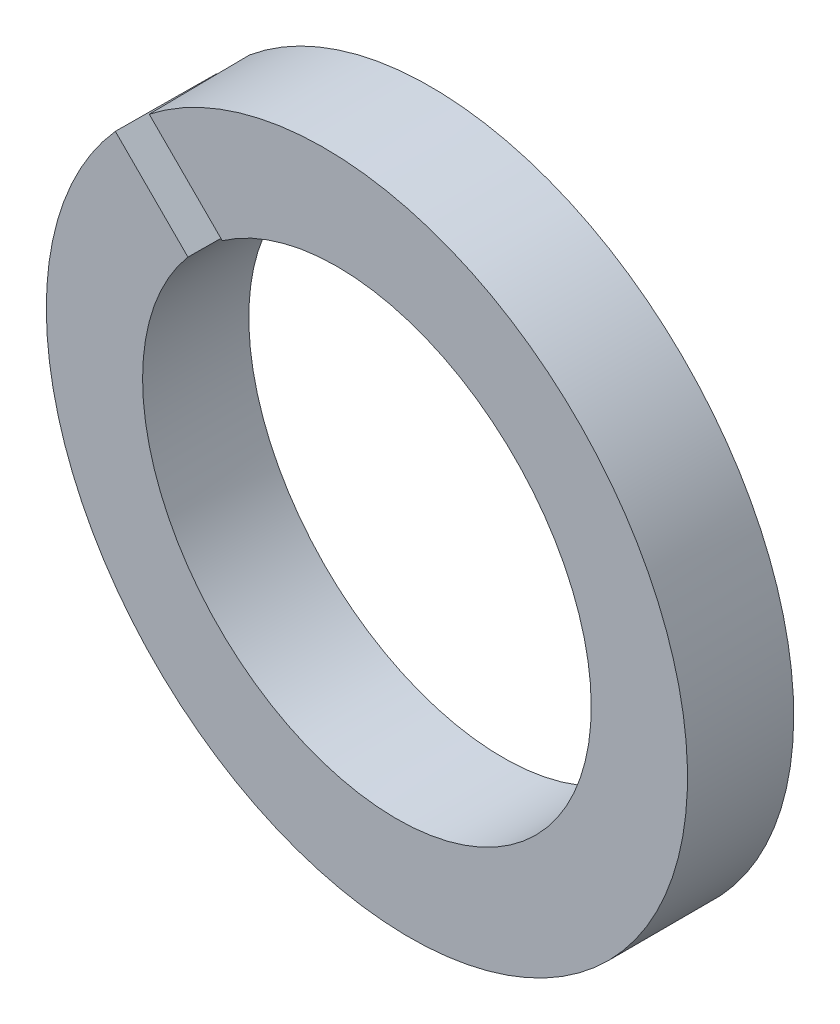
from build123d import *

# Parameters (mm, degrees)
BASE_EXTRUDE_DEPTH      = 0.001
BASE_EXTRUDE_DEPTH_BACK = 0.001
SKETCH6_W               = 2.905
SKETCH6_H               = 3.96
SKETCH8_R               = 10.003955179
SKETCH8_R_2             = 7
BOSS_EXTRUDE1_DEPTH     = 2.945
CUT_EXTRUDE1_DEPTH      = 15.963360846
CUT_EXTRUDE1_DEPTH_BACK = 15.963360846


with BuildPart() as part:
    # Sketch6 → Base-Extrude (new, two sides: drawn at the far end of the back side and taken through both)
    with BuildSketch(Plane(origin=(-4.242640687, 4.242640687, 3.255), x_dir=(0.060826394912022484, 0.060826394912020985, -0.9962932797946665), z_dir=(0.7044857341934017, 0.7044857341933883, 0.08602151263484296)).offset(-BASE_EXTRUDE_DEPTH_BACK)):
        with Locations((1.4725, 2)):
            Rectangle(SKETCH6_W, SKETCH6_H)
    extrude(amount=BASE_EXTRUDE_DEPTH + BASE_EXTRUDE_DEPTH_BACK)

    # Sketch8 → Boss-Extrude1 (add)
    with BuildSketch(Plane(origin=(-0.196039494, -0.196039494, 3.210988109), x_dir=(0.9981483386916642, -0.003915635910269119, 0.06070059112141398), z_dir=(-0.060826394912022415, -0.0608263949120211, 0.9962932797946664))):
        with Locations(Location((0, 0, 0), (0, 0, 0.224766173))):
            Circle(SKETCH8_R)
        with Locations(Location((0, 0, 0), (0, 0, 0.224766173))):
            Circle(SKETCH8_R_2, mode=Mode.SUBTRACT)
    extrude(amount=-BOSS_EXTRUDE1_DEPTH)

    # Sketch9 → Cut-Extrude1 (cut, two sides: drawn at the far end of the back side and taken through both)
    with BuildSketch(Plane.XY.offset(-CUT_EXTRUDE1_DEPTH_BACK)):
        Polygon((-34.702943681, 35.798959192), (0.298841987, 0.797173523), (-0.797173523, -0.298841987), (-36.894974703, 35.798959192), align=None)
    extrude(amount=CUT_EXTRUDE1_DEPTH + CUT_EXTRUDE1_DEPTH_BACK, mode=Mode.SUBTRACT)


solid = part.part
